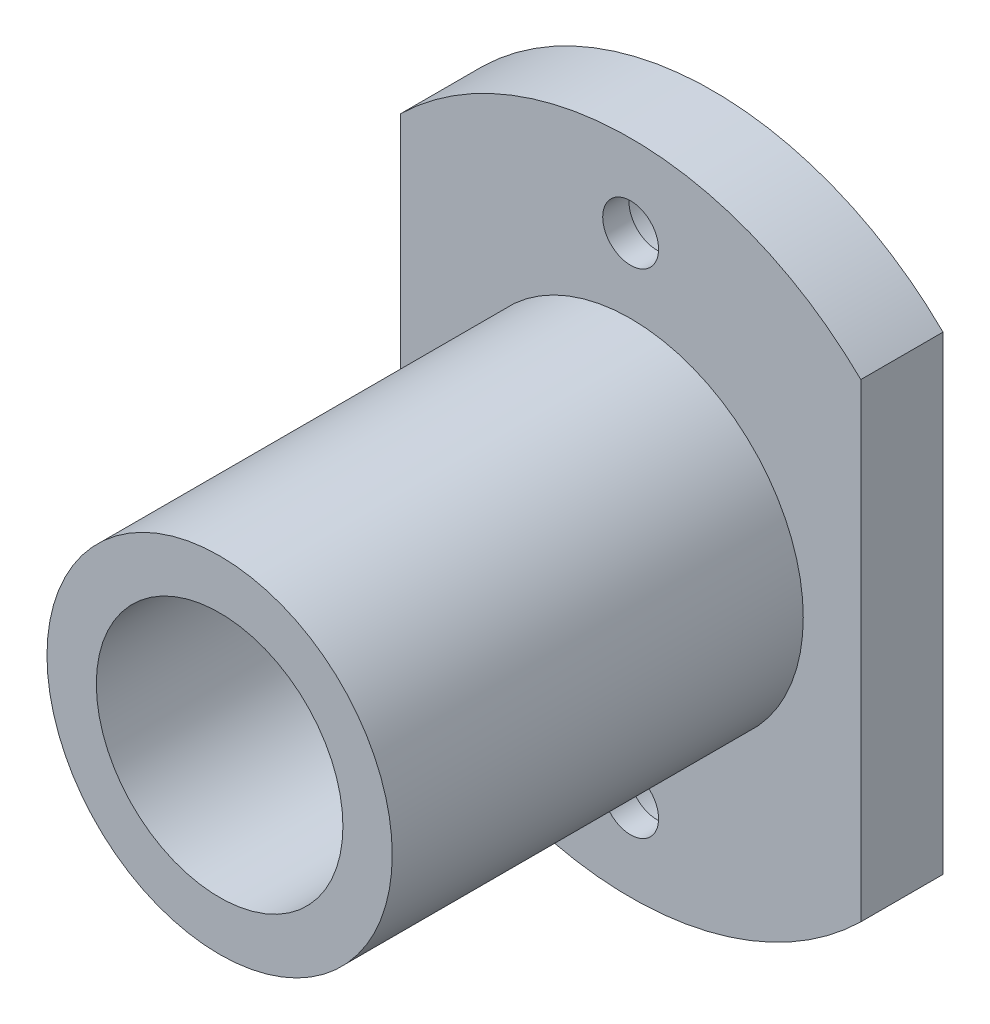
from build123d import *
from build123d.topology import SkipClean

# Parameters (mm, degrees)
SKETCH_1_R                = 10.5
SKETCH_1_R_2              = 7.5
EXTRUDE_1_DEPTH           = 25
EXTRUDE_START             = 5
SKETCH_3_R                = 20
SKETCH_3_R_2              = 7.5
EXTRUDE_3_DEPTH           = 5
HOLE_WIZARD_1_D           = 3.4
HOLE_WIZARD_1_CBORE_D     = 6
HOLE_WIZARD_1_CBORE_DEPTH = 3.4
SKETCH_6_W                = 10.726446136
SKETCH_6_H                = 40.511488533
SKETCH_6_W_2              = 7.853290921
SKETCH_6_H_2              = 42.714240865
CUT_EXTRUDE_1_DEPTH       = 10


with BuildPart() as part:
    # 草图1 → 凸台-拉伸1 (new body)
    with BuildSketch(Plane.XY):
        Circle(SKETCH_1_R)
        Circle(SKETCH_1_R_2, mode=Mode.SUBTRACT)
    extrude(amount=EXTRUDE_1_DEPTH)

    # 草图3 → 凸台-拉伸3 (add)
    with SkipClean():  # the faces are left unmerged after this step: merging them gives an invalid solid
        with BuildSketch(Plane(origin=(0, 0, 0), x_dir=(-1, 0, 0), z_dir=(0, 0, -1)).offset(EXTRUDE_START)):
            Circle(SKETCH_3_R)
            Circle(SKETCH_3_R_2, mode=Mode.SUBTRACT)
        extrude(amount=-EXTRUDE_3_DEPTH)

    # 打孔尺寸根据内六角圆柱头螺钉的类型1 (through all)
    with Locations(Plane(origin=(0, 0, -5), x_dir=(-1, 0, 0), z_dir=(0, 0, -1))):
        with Locations((0, 15), (0, -15)):
            CounterBoreHole(HOLE_WIZARD_1_D / 2, HOLE_WIZARD_1_CBORE_D / 2, HOLE_WIZARD_1_CBORE_DEPTH)

    # 草图6 → 切除-拉伸1 (cut)
    with SkipClean():  # the faces are left unmerged after this step: merging them gives an invalid solid
        with BuildSketch(Plane(origin=(0, 0, -5), x_dir=(-1, 0, 0), z_dir=(0, 0, -1))):
            with Locations((-19.363223068, 2.337558383)):
                Rectangle(SKETCH_6_W, SKETCH_6_H)
            with Locations((17.926645461, -0.870798275)):
                Rectangle(SKETCH_6_W_2, SKETCH_6_H_2)
        extrude(amount=-CUT_EXTRUDE_1_DEPTH, mode=Mode.SUBTRACT)


solid = part.part
